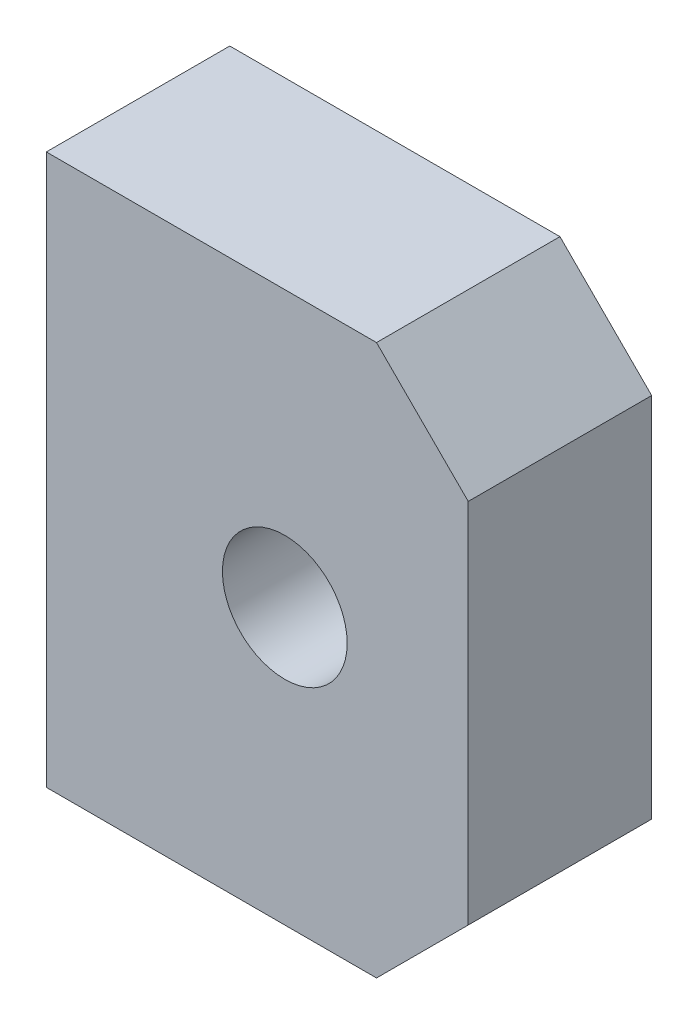
from build123d import *

# Parameters (mm, degrees)
SKETCH_1_W         = 23
SKETCH_1_H         = 30
EXTRUDE_1_DEPTH    = 10
CHAMFER_1_SIZE     = 5
HOLE_WIZARD_M8_1_D = 6.8


with BuildPart() as part:
    # 草图1 → 凸台-拉伸1 (new body)
    with BuildSketch(Plane.XY):
        Rectangle(SKETCH_1_W, SKETCH_1_H)
    extrude(amount=EXTRUDE_1_DEPTH)

    # 倒角1
    chamfer_1_edges = [part.edges().sort_by_distance(p)[0] for p in [
        (11.5, 15, 5),
        (11.5, -15, 5),
    ]]
    chamfer(chamfer_1_edges, length=CHAMFER_1_SIZE)

    # M8 螺纹孔1 (through all)
    with Locations(Plane(origin=(0, 0, 0), x_dir=(-1, 0, 0), z_dir=(0, 0, -1))):
        with Locations((-1.5, 0)):
            Hole(HOLE_WIZARD_M8_1_D / 2)


solid = part.part
